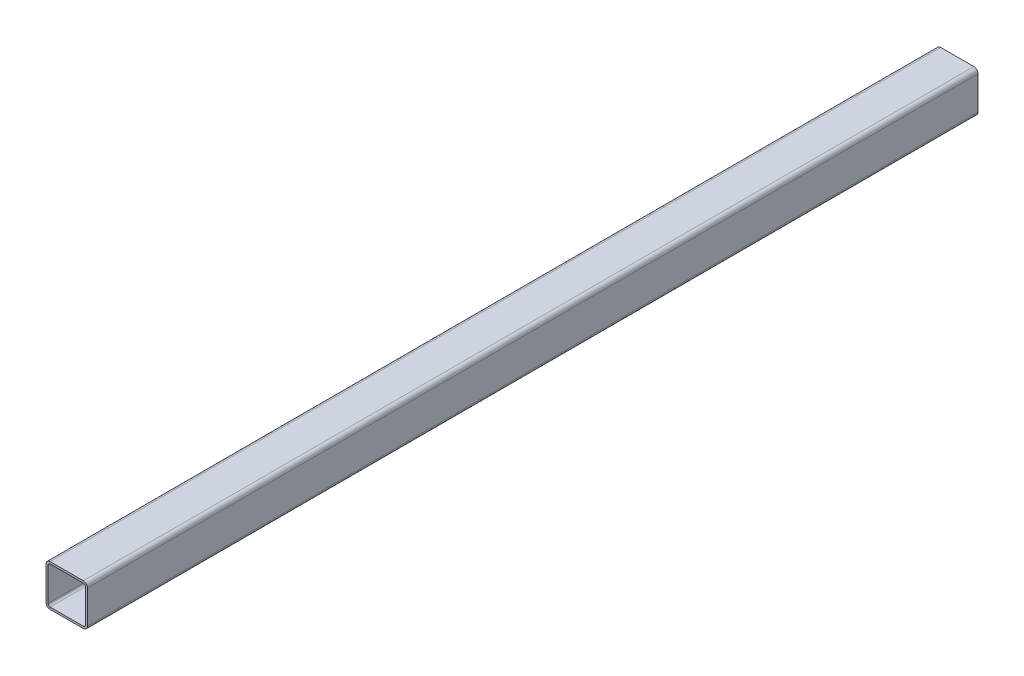
SolidWorks part; units mm, degrees
material "Q235A"
ref_plane "Front Plane" through (0, 0, 0) normal (0, 0, 1) x (1, 0, 0)
ref_plane "Top Plane" through (0, 0, 0) normal (0, 1, 0) x (1, 0, 0)
ref_plane "Right Plane" through (0, 0, 0) normal (1, 0, 0) x (0, 0, -1)
sketch "Sketch1" plane through (0, 0, 0) normal (0, 0, 1) x (1, 0, 0)
  line L1 (-20, 20) -> (20, 20)
  line L2 (-20, 20) -> (-20, -20)
  line L3 (-20, -20) -> (20, -20)
  line L4 (20, 20) -> (20, -20)
  line L5 (-20, 20) -> (20, -20) construction
  line L6 (-20, -20) -> (20, 20) construction
  line L7 (-18, 18) -> (18, 18)
  line L8 (-18, 18) -> (-18, -18)
  line L9 (-18, -18) -> (18, -18)
  line L10 (18, 18) -> (18, -18)
  line L11 (-18, 18) -> (18, -18) construction
  line L12 (-18, -18) -> (18, 18) construction
  point P0 (0, 0)
  point P6 (0, 0)
  dimension "D1" = 40
  dimension "D2" = 40
  dimension "D3" = 2
  dimension "D4" = 2
extrude "Boss-Extrude1" add sketch "Sketch1" along normal blind 860
fillet "Fillet1" radius 2 4 edges at (18, 18, 430) (-18, 18, 430) (-18, -18, 430) (18, -18, 430)
fillet "Fillet2" radius 4 4 edges at (20, 20, 430) (20, -20, 430) (-20, 20, 430) (-20, -20, 430)
